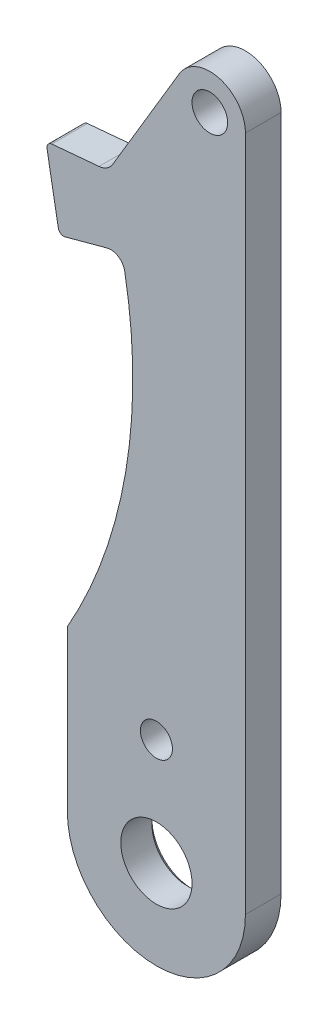
SolidWorks part; units mm, degrees
material "Q235B"
ref_plane "Front" through (0, 0, 0) normal (0, 0, 1) x (1, 0, 0)
ref_plane "Top" through (0, 0, 0) normal (0, 1, 0) x (1, 0, 0)
ref_plane "Right" through (0, 0, 0) normal (1, 0, 0) x (0, 0, -1)
sketch "Sketch1" plane through (0, 0, 0) normal (0, 0, 1) x (1, 0, 0)
  line L0 (0, 105.0188) -> (0, -84.8422) construction
  line L4 (0, 0) -> (363.8961, 0) construction
  line L6 (-54.5, 278) -> (-62, 320)
  line L8 (-62, 320) -> (-27.1399, 323.1263)
  line L9 (-54.5, 278) -> (-27.7651, 285.226)
  line L10 (0, 60) -> (0, 0) construction
  line L11 (50, 0) -> (50, 380)
  line L12 (-27.1399, 323.1263) -> (12.8154, 390.2319)
  line L15 (-50, 0) -> (-50, 90)
  arc A0 (50, 380) -> (12.8154, 390.2319) centre (30, 380) ccw
  arc A1 (-50, 0) -> (50, 0) centre (0, 0) ccw
  circle A4 centre (0, 60) radius 9
  circle A5 centre (30, 380) radius 10
  arc A6 (-17.8077, 278.9397) -> (-27.7651, 285.226) centre (-25.6777, 277.5031) ccw
  circle A7 centre (0, 0) radius 20
  circle A8 centre (0, 0) radius 30 construction
  arc A9 (50, 0) -> (-50, 0) centre (0, 0) ccw construction
  arc A10 (-50, 90) -> (-17.8077, 278.9397) centre (-293.2563, 228.6593) ccw
  point P13 (-19.5, 287.4599)
  dimension "D4" = 112
  dimension "D5" = 20
  dimension "D6" = 35
  dimension "D7" = 50
  dimension "D8" = 18
  dimension "D14" = 278
  dimension "D15" = 20
  dimension "D16" = 40
  dimension "D9" = 60
  dimension "D19" = 8
  dimension "D3" = 287.4599
  dimension "D26" = 63.2563
  dimension "D13" = 280
  dimension "D17" = 60
  dimension "D10" = 380
  dimension "D11" = 320
  dimension "D12" = 35
  dimension "D20" = 104.5
  dimension "D22" = 27.6943
  dimension "D23" = 85
  dimension "D24" = 85
  dimension "D25" = 42.6644
  dimension "D28" = 90
  dimension "D31" = 56.8737
extrude "Extrude1" add sketch "Sketch1" along normal blind 20
fillet "Fillet1" radius 3 2 edges at (-62, 320, 10) (-54.5, 278, 10)
fillet "Fillet2" radius 10 1 edges at (-27.1399, 323.1263, 10)
chamfer "Chamfer1" distance 2.5 angle 45 1 edges at (20, 0, 0)
